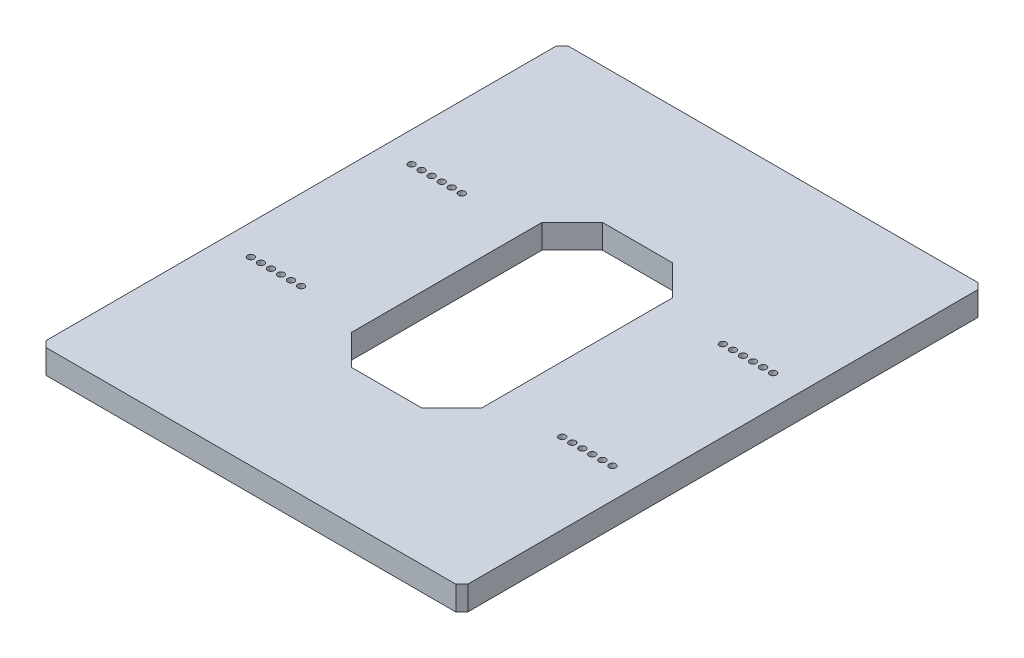
from build123d import *

# Parameters (mm, degrees)
SKETCH_1_W                   = 210
SKETCH_1_H                   = 260
EXTRUDE_1_DEPTH              = 12
HOLE_WIZARD_M4_1_D           = 3.3
HOLE_WIZARD_M4_1_CSINK_D     = 4.05
HOLE_WIZARD_M4_1_CSINK_ANGLE = 90
PATTERN_LINEAR_1_COUNT       = 6
PATTERN_LINEAR_1_PITCH       = 5
MIRROR_1_COPY_1_D            = 3.3
MIRROR_1_COPY_1_CSINK_D      = 4.05
MIRROR_1_COPY_1_CSINK_ANGLE  = 90
MIRROR_1_COPY_2_D            = 3.3
MIRROR_1_COPY_2_CSINK_D      = 4.05
MIRROR_1_COPY_2_CSINK_ANGLE  = 90
MIRROR_1_COPY_3_D            = 3.3
MIRROR_1_COPY_3_CSINK_D      = 4.05
MIRROR_1_COPY_3_CSINK_ANGLE  = 90
MIRROR_1_COPY_4_D            = 3.3
MIRROR_1_COPY_4_CSINK_D      = 4.05
MIRROR_1_COPY_4_CSINK_ANGLE  = 90
MIRROR_1_COPY_5_D            = 3.3
MIRROR_1_COPY_5_CSINK_D      = 4.05
MIRROR_1_COPY_5_CSINK_ANGLE  = 90
MIRROR_2_COPY_1_D            = 3.3
MIRROR_2_COPY_1_CSINK_D      = 4.05
MIRROR_2_COPY_1_CSINK_ANGLE  = 90
MIRROR_2_COPY_2_D            = 3.3
MIRROR_2_COPY_2_CSINK_D      = 4.05
MIRROR_2_COPY_2_CSINK_ANGLE  = 90
MIRROR_2_COPY_3_D            = 3.3
MIRROR_2_COPY_3_CSINK_D      = 4.05
MIRROR_2_COPY_3_CSINK_ANGLE  = 90
MIRROR_2_COPY_4_D            = 3.3
MIRROR_2_COPY_4_CSINK_D      = 4.05
MIRROR_2_COPY_4_CSINK_ANGLE  = 90
MIRROR_2_COPY_5_D            = 3.3
MIRROR_2_COPY_5_CSINK_D      = 4.05
MIRROR_2_COPY_5_CSINK_ANGLE  = 90
MIRROR_2_COPY_6_D            = 3.3
MIRROR_2_COPY_6_CSINK_D      = 4.05
MIRROR_2_COPY_6_CSINK_ANGLE  = 90
MIRROR_2_COPY_7_D            = 3.3
MIRROR_2_COPY_7_CSINK_D      = 4.05
MIRROR_2_COPY_7_CSINK_ANGLE  = 90
MIRROR_2_COPY_8_D            = 3.3
MIRROR_2_COPY_8_CSINK_D      = 4.05
MIRROR_2_COPY_8_CSINK_ANGLE  = 90
MIRROR_2_COPY_9_D            = 3.3
MIRROR_2_COPY_9_CSINK_D      = 4.05
MIRROR_2_COPY_9_CSINK_ANGLE  = 90
MIRROR_2_COPY_10_D           = 3.3
MIRROR_2_COPY_10_CSINK_D     = 4.05
MIRROR_2_COPY_10_CSINK_ANGLE = 90
MIRROR_2_COPY_11_D           = 3.3
MIRROR_2_COPY_11_CSINK_D     = 4.05
MIRROR_2_COPY_11_CSINK_ANGLE = 90
CHAMFER_1_SIZE               = 3
CUT_EXTRUDE_1_REACH          = 169.538
SKETCH_3_W                   = 65
SKETCH_3_H                   = 125
CHAMFER_2_SIZE               = 15


with BuildPart() as part:
    # 草图1 → 凸台-拉伸1 (new body)
    with BuildSketch(Plane(origin=(0, 0, 0), x_dir=(1, 0, 0), z_dir=(0, 1, 0))):
        Rectangle(SKETCH_1_W, SKETCH_1_H)
    extrude(amount=EXTRUDE_1_DEPTH)

    # M4 螺纹孔1 (through all)
    with Locations(Plane(origin=(-90, 0, -40), x_dir=(0, 0, -1), z_dir=(0, -1, 0))):
        with Locations((0, 0)):
            hole_wizard_m4_1 = CounterSinkHole(HOLE_WIZARD_M4_1_D / 2, HOLE_WIZARD_M4_1_CSINK_D / 2, counter_sink_angle=HOLE_WIZARD_M4_1_CSINK_ANGLE)

    # 阵列(线性)1: M4 螺纹孔1 ×6
    with Locations(*[(i * PATTERN_LINEAR_1_PITCH, 0, 0) for i in range(1, PATTERN_LINEAR_1_COUNT)]):
        add(hole_wizard_m4_1, mode=Mode.SUBTRACT)

    # 镜向1: M4 螺纹孔1 across plane
    add(hole_wizard_m4_1.mirror(Plane(origin=(0, 0, 0), x_dir=(0, 0, 1), z_dir=(1, 0, 0))), mode=Mode.SUBTRACT)

    # 镜向1 copy 1 (through all)
    with Locations(Plane(origin=(85, 0, -40), x_dir=(0, 0, -1), z_dir=(0, -1, 0))):
        with Locations((0, 0)):
            CounterSinkHole(MIRROR_1_COPY_1_D / 2, MIRROR_1_COPY_1_CSINK_D / 2, counter_sink_angle=MIRROR_1_COPY_1_CSINK_ANGLE)

    # 镜向1 copy 2 (through all)
    with Locations(Plane(origin=(80, 0, -40), x_dir=(0, 0, -1), z_dir=(0, -1, 0))):
        with Locations((0, 0)):
            CounterSinkHole(MIRROR_1_COPY_2_D / 2, MIRROR_1_COPY_2_CSINK_D / 2, counter_sink_angle=MIRROR_1_COPY_2_CSINK_ANGLE)

    # 镜向1 copy 3 (through all)
    with Locations(Plane(origin=(75, 0, -40), x_dir=(0, 0, -1), z_dir=(0, -1, 0))):
        with Locations((0, 0)):
            CounterSinkHole(MIRROR_1_COPY_3_D / 2, MIRROR_1_COPY_3_CSINK_D / 2, counter_sink_angle=MIRROR_1_COPY_3_CSINK_ANGLE)

    # 镜向1 copy 4 (through all)
    with Locations(Plane(origin=(70, 0, -40), x_dir=(0, 0, -1), z_dir=(0, -1, 0))):
        with Locations((0, 0)):
            CounterSinkHole(MIRROR_1_COPY_4_D / 2, MIRROR_1_COPY_4_CSINK_D / 2, counter_sink_angle=MIRROR_1_COPY_4_CSINK_ANGLE)

    # 镜向1 copy 5 (through all)
    with Locations(Plane(origin=(65, 0, -40), x_dir=(0, 0, -1), z_dir=(0, -1, 0))):
        with Locations((0, 0)):
            CounterSinkHole(MIRROR_1_COPY_5_D / 2, MIRROR_1_COPY_5_CSINK_D / 2, counter_sink_angle=MIRROR_1_COPY_5_CSINK_ANGLE)

    # 镜向2: M4 螺纹孔1 across plane
    add(hole_wizard_m4_1.mirror(Plane.XY), mode=Mode.SUBTRACT)

    # 镜向2 copy 1 (through all)
    with Locations(Plane(origin=(-85, 0, 40), x_dir=(0, 0, 1), z_dir=(0, -1, 0))):
        with Locations((0, 0)):
            CounterSinkHole(MIRROR_2_COPY_1_D / 2, MIRROR_2_COPY_1_CSINK_D / 2, counter_sink_angle=MIRROR_2_COPY_1_CSINK_ANGLE)

    # 镜向2 copy 2 (through all)
    with Locations(Plane(origin=(-80, 0, 40), x_dir=(0, 0, 1), z_dir=(0, -1, 0))):
        with Locations((0, 0)):
            CounterSinkHole(MIRROR_2_COPY_2_D / 2, MIRROR_2_COPY_2_CSINK_D / 2, counter_sink_angle=MIRROR_2_COPY_2_CSINK_ANGLE)

    # 镜向2 copy 3 (through all)
    with Locations(Plane(origin=(-75, 0, 40), x_dir=(0, 0, 1), z_dir=(0, -1, 0))):
        with Locations((0, 0)):
            CounterSinkHole(MIRROR_2_COPY_3_D / 2, MIRROR_2_COPY_3_CSINK_D / 2, counter_sink_angle=MIRROR_2_COPY_3_CSINK_ANGLE)

    # 镜向2 copy 4 (through all)
    with Locations(Plane(origin=(-70, 0, 40), x_dir=(0, 0, 1), z_dir=(0, -1, 0))):
        with Locations((0, 0)):
            CounterSinkHole(MIRROR_2_COPY_4_D / 2, MIRROR_2_COPY_4_CSINK_D / 2, counter_sink_angle=MIRROR_2_COPY_4_CSINK_ANGLE)

    # 镜向2 copy 5 (through all)
    with Locations(Plane(origin=(-65, 0, 40), x_dir=(0, 0, 1), z_dir=(0, -1, 0))):
        with Locations((0, 0)):
            CounterSinkHole(MIRROR_2_COPY_5_D / 2, MIRROR_2_COPY_5_CSINK_D / 2, counter_sink_angle=MIRROR_2_COPY_5_CSINK_ANGLE)

    # 镜向2 copy 6 (through all)
    with Locations(Plane(origin=(90, 0, 40), x_dir=(0, 0, 1), z_dir=(0, -1, 0))):
        with Locations((0, 0)):
            CounterSinkHole(MIRROR_2_COPY_6_D / 2, MIRROR_2_COPY_6_CSINK_D / 2, counter_sink_angle=MIRROR_2_COPY_6_CSINK_ANGLE)

    # 镜向2 copy 7 (through all)
    with Locations(Plane(origin=(85, 0, 40), x_dir=(0, 0, 1), z_dir=(0, -1, 0))):
        with Locations((0, 0)):
            CounterSinkHole(MIRROR_2_COPY_7_D / 2, MIRROR_2_COPY_7_CSINK_D / 2, counter_sink_angle=MIRROR_2_COPY_7_CSINK_ANGLE)

    # 镜向2 copy 8 (through all)
    with Locations(Plane(origin=(80, 0, 40), x_dir=(0, 0, 1), z_dir=(0, -1, 0))):
        with Locations((0, 0)):
            CounterSinkHole(MIRROR_2_COPY_8_D / 2, MIRROR_2_COPY_8_CSINK_D / 2, counter_sink_angle=MIRROR_2_COPY_8_CSINK_ANGLE)

    # 镜向2 copy 9 (through all)
    with Locations(Plane(origin=(75, 0, 40), x_dir=(0, 0, 1), z_dir=(0, -1, 0))):
        with Locations((0, 0)):
            CounterSinkHole(MIRROR_2_COPY_9_D / 2, MIRROR_2_COPY_9_CSINK_D / 2, counter_sink_angle=MIRROR_2_COPY_9_CSINK_ANGLE)

    # 镜向2 copy 10 (through all)
    with Locations(Plane(origin=(70, 0, 40), x_dir=(0, 0, 1), z_dir=(0, -1, 0))):
        with Locations((0, 0)):
            CounterSinkHole(MIRROR_2_COPY_10_D / 2, MIRROR_2_COPY_10_CSINK_D / 2, counter_sink_angle=MIRROR_2_COPY_10_CSINK_ANGLE)

    # 镜向2 copy 11 (through all)
    with Locations(Plane(origin=(65, 0, 40), x_dir=(0, 0, 1), z_dir=(0, -1, 0))):
        with Locations((0, 0)):
            CounterSinkHole(MIRROR_2_COPY_11_D / 2, MIRROR_2_COPY_11_CSINK_D / 2, counter_sink_angle=MIRROR_2_COPY_11_CSINK_ANGLE)

    # 倒角1
    chamfer_1_edges = [part.edges().sort_by_distance(p)[0] for p in [
        (105, 6, 130),
        (-105, 6, 130),
        (-105, 6, -130),
        (105, 6, -130),
    ]]
    chamfer(chamfer_1_edges, length=CHAMFER_1_SIZE)

    # 草图3 → 切除-拉伸1 (cut, up to next)
    with BuildSketch(Plane.XZ, mode=Mode.PRIVATE) as cut_extrude_1_sk1:
        Rectangle(SKETCH_3_W, SKETCH_3_H)
    cut_extrude_1_tool1 = extrude(cut_extrude_1_sk1.sketch, amount=-CUT_EXTRUDE_1_REACH, mode=Mode.PRIVATE) & part.part
    add(cut_extrude_1_tool1.solids().sort_by_distance((0, 0, 0))[0], mode=Mode.SUBTRACT)

    # 倒角2
    chamfer_2_edges = [part.edges().sort_by_distance(p)[0] for p in [
        (-32.5, 6, -62.5),
        (-32.5, 6, 62.5),
        (32.5, 6, 62.5),
        (32.5, 6, -62.5),
    ]]
    chamfer(chamfer_2_edges, length=CHAMFER_2_SIZE)


solid = part.part
